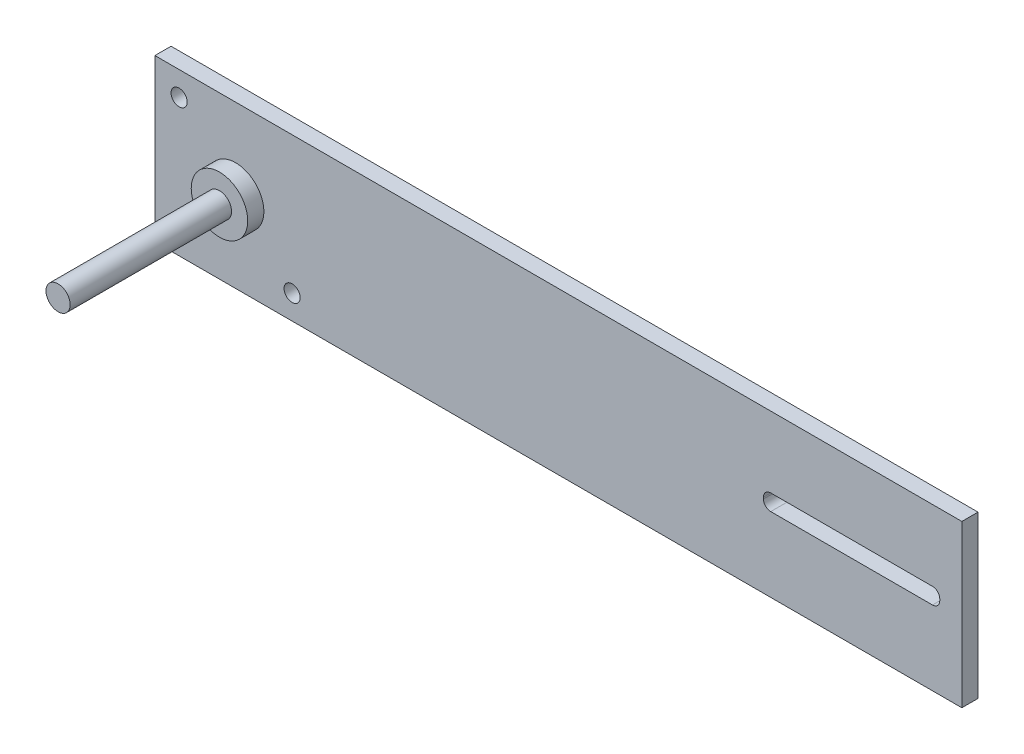
SolidWorks part; units mm, degrees
material "PVC Rigid"
ref_plane "Front Plane" through (0, 0, 0) normal (0, 0, 1) x (1, 0, 0)
ref_plane "Top Plane" through (0, 0, 0) normal (0, 1, 0) x (1, 0, 0)
ref_plane "Right Plane" through (0, 0, 0) normal (1, 0, 0) x (0, 0, -1)
sketch "Sketch1" plane through (0, 0, 0) normal (0, 0, 1) x (1, 0, 0)
  line L1 (250, 50) -> (-250, 50)
  line L2 (250, 50) -> (250, -50)
  line L3 (250, -50) -> (-250, -50)
  line L4 (-250, 50) -> (-250, -50)
  line L5 (250, 50) -> (-250, -50) construction
  line L6 (250, -50) -> (-250, 50) construction
  point P0 (0, 0)
  dimension "D1" = 500
  dimension "D2" = 100
extrude "Boss-Extrude1" add sketch "Sketch1" along normal blind 10
sketch "Sketch3" plane through (0, 0, 10) normal (0, 0, 1) x (1, 0, 0)
  line L0 (240.6687, 1.0678) -> (68.4223, 1.0678) construction
  line L1 (231.805, -3.9322) -> (131.5582, -3.9322)
  line L2 (236.305, 0.5678) -> (236.305, 1.5678)
  line L3 (231.805, 6.0678) -> (131.5582, 6.0678)
  line L4 (127.0582, 0.5678) -> (127.0582, 1.5678)
  line L5 (236.305, -3.9322) -> (127.0582, 6.0678) construction
  line L6 (236.305, 6.0678) -> (127.0582, -3.9322) construction
  arc A0 (236.305, 1.5678) -> (231.805, 6.0678) centre (231.805, 1.5678) ccw
  arc A1 (231.805, -3.9322) -> (236.305, 0.5678) centre (231.805, 0.5678) ccw
  arc A2 (131.5582, -3.9322) -> (127.0582, 0.5678) centre (131.5582, 0.5678) cw
  arc A3 (127.0582, 1.5678) -> (131.5582, 6.0678) centre (131.5582, 1.5678) cw
  point P0 (181.6816, 1.0678)
  dimension "D2" = 4.5
  dimension "D1" = 10
extrude "Cut-Extrude1" cut sketch "Sketch3" against normal blind 60
sketch "Sketch4" plane through (0, 0, 10) normal (0, 0, 1) x (1, 0, 0)
  line L0 (-250, 50) -> (-150, -50) construction
  line L1 (-250, -50) -> (250, -50) construction
  line L2 (-250, 0) -> (-138.7263, 0) construction
  line L3 (-250, 50) -> (-250, -50) construction
  line L4 (250, 50) -> (-250, 50) construction
  circle A0 centre (-235, 35) radius 5
  circle A1 centre (-165, -35) radius 5
  dimension "D1" = 10
  dimension "D2" = 10
  dimension "D3" = 15
  dimension "D4" = 15
  dimension "D5" = 45
extrude "Cut-Extrude2" cut sketch "Sketch4" against normal blind 60
sketch "Sketch2" plane through (0, 0, 10) normal (0, 0, 1) x (1, 0, 0)
  line L0 (-250, 50) -> (-150, -50) construction
  line L1 (-250, -50) -> (250, -50) construction
  line L2 (-250, 50) -> (-250, -50) construction
  circle A0 centre (-200, 0) radius 17.5
  dimension "D1" = 35
  dimension "D2" = 45
extrude "Boss-Extrude2" add sketch "Sketch2" along normal blind 60
sketch "Sketch5" plane through (0, 0, 70) normal (0, 0, 1) x (1, 0, 0)
  circle A0 centre (-200, 0) radius 17.5
  circle A1 centre (-200, 0) radius 7.5
  dimension "D1" = 15
extrude "Cut-Extrude3" cut sketch "Sketch5" against normal blind 50
sketch "Sketch6" plane through (0, 0, 70) normal (0, 0, 1) x (1, 0, 0)
  circle A0 centre (-200, 0) radius 7.5
extrude "Boss-Extrude3" add sketch "Sketch6" along normal blind 50
